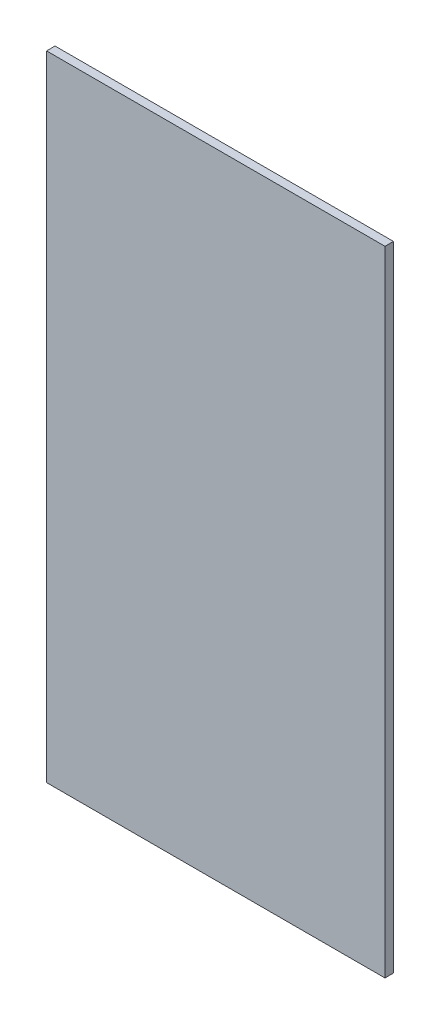
SolidWorks part; units mm, degrees
material "普通碳钢"
ref_plane "Front Plane" through (0, 0, 0) normal (0, 0, 1) x (1, 0, 0)
ref_plane "Top Plane" through (0, 0, 0) normal (0, 1, 0) x (1, 0, 0)
ref_plane "Right Plane" through (0, 0, 0) normal (1, 0, 0) x (0, 0, -1)
sketch "Sketch1" plane through (0, 0, 0) normal (0, 0, 1) x (1, 0, 0)
  line L1 (-200, 374.5) -> (200, 374.5)
  line L2 (-200, 374.5) -> (-200, -374.5)
  line L3 (-200, -374.5) -> (200, -374.5)
  line L4 (200, 374.5) -> (200, -374.5)
  dimension "D1" = 749
  dimension "D2" = 400
  dimension "D3" = 374.5
  dimension "D4" = 200
extrude "Boss-Extrude1" add sketch "Sketch1" along normal mid plane 10
